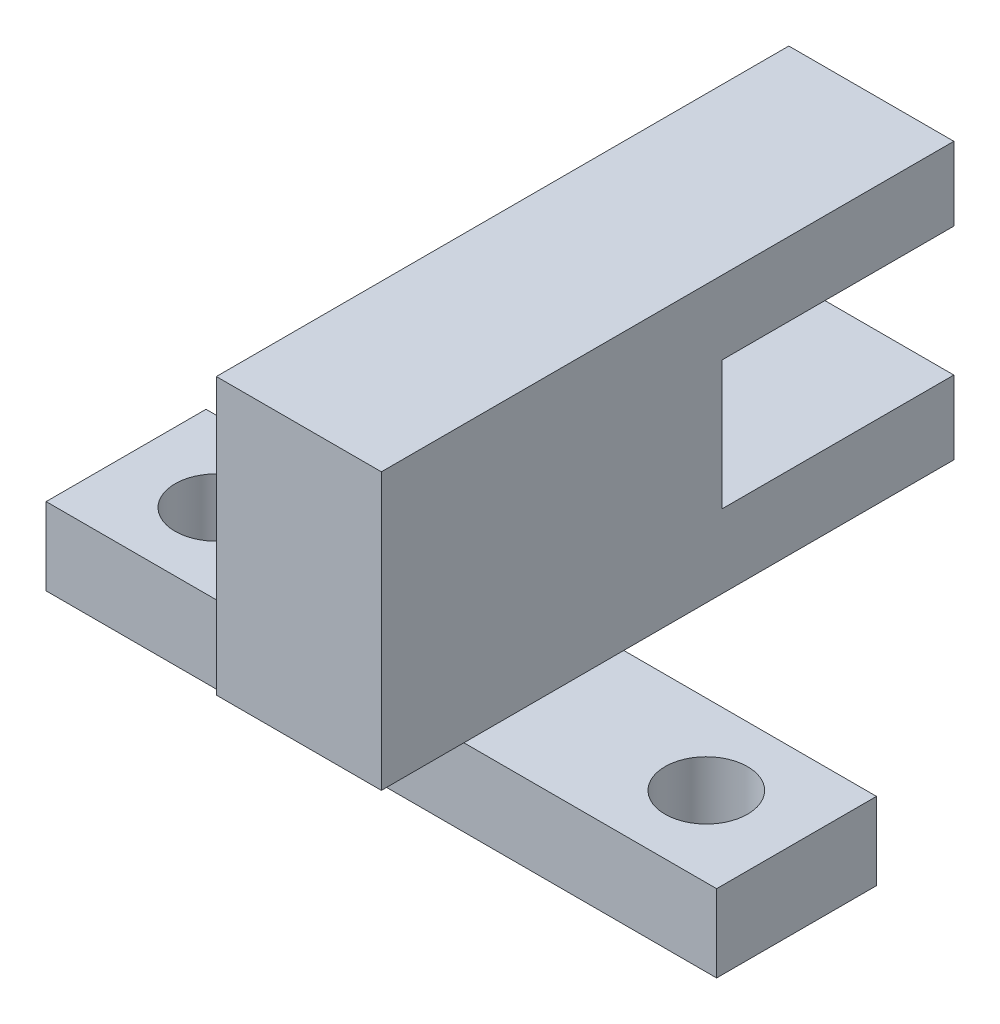
from build123d import *

# Parameters (mm, degrees)
SKETCH_1_W          = 26
SKETCH_1_H          = 6.2
EXTRUDE_1_DEPTH     = 3
SKETCH_2_W          = 6.4
SKETCH_2_H          = 22.2
EXTRUDE_2_DEPTH     = 10.7
SKETCH_3_W          = 9
SKETCH_3_H          = 5
CUT_EXTRUDE_1_DEPTH = 10.7
SKETCH_4_R          = 1.6
CUT_EXTRUDE_2_DEPTH = 10.7


with BuildPart() as part:
    # 草图1 → 凸台-拉伸1 (new body)
    with BuildSketch(Plane(origin=(0, 0, 0), x_dir=(1, 0, 0), z_dir=(0, 1, 0))):
        Rectangle(SKETCH_1_W, SKETCH_1_H)
    extrude(amount=EXTRUDE_1_DEPTH)

    # 草图2 → 凸台-拉伸2 (add)
    with BuildSketch(Plane(origin=(0, 3, 0), x_dir=(1, 0, 0), z_dir=(0, 1, 0))):
        with Locations((0, 4.8)):
            Rectangle(SKETCH_2_W, SKETCH_2_H)
    extrude(amount=EXTRUDE_2_DEPTH)

    # 草图3 → 切除-拉伸1 (cut)
    with BuildSketch(Plane.ZY.offset(3.2)):
        with Locations((-11.4, 8.35)):
            Rectangle(SKETCH_3_W, SKETCH_3_H)
    extrude(amount=-CUT_EXTRUDE_1_DEPTH, mode=Mode.SUBTRACT)

    # 草图4 → 切除-拉伸2 (cut)
    with BuildSketch(Plane(origin=(0, 3, 0), x_dir=(1, 0, 0), z_dir=(0, 1, 0))):
        with Locations(Location((-9.5, 0, 0), (0, 0, 270))):
            Circle(SKETCH_4_R)
        with Locations(Location((9.5, 0, 0), (0, 0, 270))):
            Circle(SKETCH_4_R)
    extrude(amount=-CUT_EXTRUDE_2_DEPTH, mode=Mode.SUBTRACT)


solid = part.part
